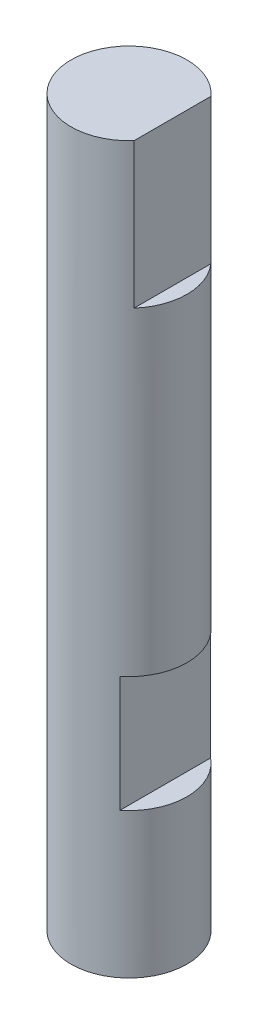
SolidWorks part; units mm, degrees
material "Q235"
ref_plane "Front" through (0, 0, 0) normal (0, 0, 1) x (1, 0, 0)
ref_plane "Top" through (0, 0, 0) normal (0, 1, 0) x (1, 0, 0)
ref_plane "Right" through (0, 0, 0) normal (1, 0, 0) x (0, 0, -1)
sketch "Sketch1" plane through (0, 0, 0) normal (0, 1, 0) x (1, 0, 0)
  circle A0 centre (0, 0) radius 8
  dimension "D1" = 16
extrude "Boss-Extrude1" add sketch "Sketch1" along normal blind 100
sketch "Sketch2" plane through (0, 0, 0) normal (0, 0, 1) x (1, 0, 0)
  line L0 (-8, 0) -> (8, 0) construction
  line L1 (8, 80) -> (6, 80)
  line L2 (8, 80) -> (8, 100)
  line L3 (8, 100) -> (6, 100)
  line L4 (6, 80) -> (6, 100)
  line L5 (8, 100) -> (-8, 100) construction
  line L6 (8, 0) -> (8, 100) construction
  line L7 (5, 36) -> (11, 36)
  line L8 (5, 36) -> (5, 20)
  line L9 (5, 20) -> (11, 20)
  line L10 (11, 36) -> (11, 20)
  line L11 (5, 36) -> (11, 20) construction
  line L12 (5, 20) -> (11, 36) construction
  point P4 (8, 28)
  dimension "D1" = 20
  dimension "D2" = 2
  dimension "D3" = 1
  dimension "D4" = 16
  dimension "D5" = 20
extrude "Cut-Extrude1" cut sketch "Sketch2" against normal through all both and the other way through all
